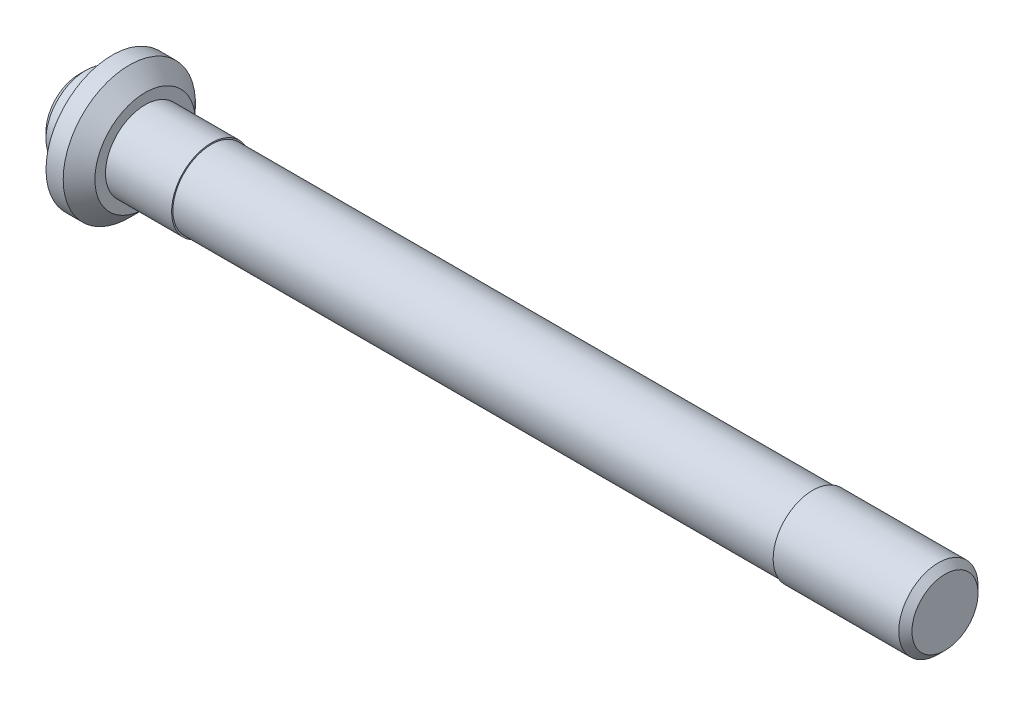
from build123d import *

# Parameters (mm, degrees)
CHAMFER1_SIZE         = 1.2
M3_TAPPED_HOLE1_D     = 2.5
M3_TAPPED_HOLE1_DEPTH = 7.5
M3_TAPPED_HOLE1_TIP   = 0.751075774
CHAMFER2_SIZE         = 0.5


with BuildPart() as part:
    # Sketch1 → Revolve1 (revolve)
    with BuildSketch(Plane.XY, mode=Mode.PRIVATE) as revolve1_sk:
        Polygon((0, 0), (0, 3), (2.5, 3), (2.5, 5), (5, 5), (5, 3), (10, 3), (10, 2.9), (55.5, 2.9), (55.5, 3), (65.5, 3), (65.5, 0), align=None)
    revolve(revolve1_sk.sketch.rotate(Axis((0, 0, 0), (1, 0, 0)), 90), axis=Axis((0, 0, 0), (1, 0, 0)))

    # Chamfer1
    chamfer1_edges = [part.edges().sort_by_distance(p)[0] for p in [
        (5, 0, -5),
    ]]
    chamfer(chamfer1_edges, length=CHAMFER1_SIZE)

    # M3 Tapped Hole1
    with Locations(Plane.ZY):
        with Locations((0, 0)):
            Hole(M3_TAPPED_HOLE1_D / 2, depth=M3_TAPPED_HOLE1_DEPTH)
            with Locations((0, 0, -(M3_TAPPED_HOLE1_DEPTH + M3_TAPPED_HOLE1_TIP / 2))):  # 118° drill point
                Cone(0, M3_TAPPED_HOLE1_D / 2, M3_TAPPED_HOLE1_TIP, mode=Mode.SUBTRACT)

    # Chamfer2
    chamfer2_edges = [part.edges().sort_by_distance(p)[0] for p in [
        (0, 0, -3),
        (65.5, 0, -3),
    ]]
    chamfer(chamfer2_edges, length=CHAMFER2_SIZE)


solid = part.part
